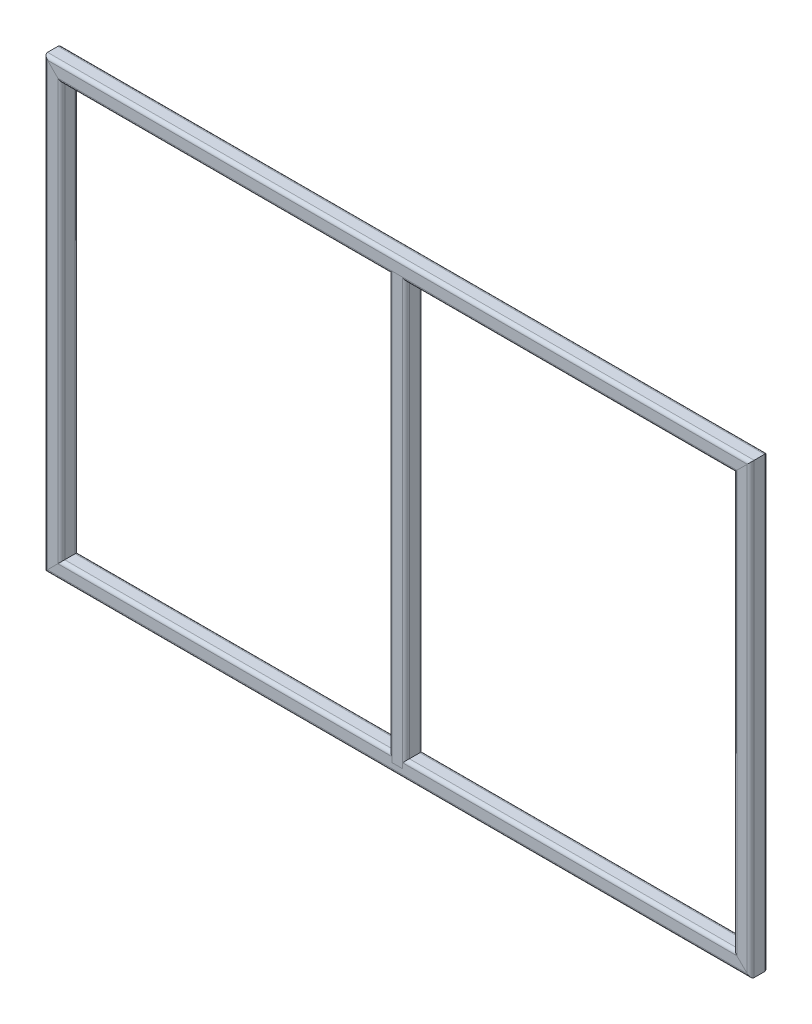
from build123d import *

# Parameters (mm, degrees)
SQUARE_TUBE_20_X_20_X_2_1_DEPTH      = 815.142135624
SQUARE_TUBE_20_X_20_X_2_1_DEPTH_BACK = 15.142135624
SQUARE_TUBE_20_X_20_X_2_1_2_DEPTH    = 530.284271247
SQUARE_TUBE_20_X_20_X_2_1_3_DEPTH    = 830.284271247
SQUARE_TUBE_20_X_20_X_2_1_4_DEPTH    = 530.284271247
SQUARE_TUBE_20_X_20_X_2_2_DEPTH      = 500


with BuildPart() as part:
    # Sketch1 → Square tube 20 X 20 X 2(1) (new, two sides: drawn at the far end of the back side and taken through both)
    with BuildSketch(Plane(origin=(-400, 250, 0), x_dir=(0, 1, 0), z_dir=(1, 0, 0)).offset(-SQUARE_TUBE_20_X_20_X_2_1_DEPTH_BACK)):
        with BuildLine():
            Line((-6, -10), (6, -10))
            ThreePointArc((6, -10), (8.828427125, -8.828427125), (10, -6))
            Line((10, -6), (10, 6))
            ThreePointArc((10, 6), (8.828427125, 8.828427125), (6, 10))
            Line((6, 10), (-6, 10))
            ThreePointArc((-6, 10), (-8.828427125, 8.828427125), (-10, 6))
            Line((-10, 6), (-10, -6))
            ThreePointArc((-10, -6), (-8.828427125, -8.828427125), (-6, -10))
        make_face()
        with BuildLine():
            Line((-6, -8), (6, -8))
            ThreePointArc((6, -8), (7.414213562, -7.414213562), (8, -6))
            Line((8, -6), (8, 6))
            ThreePointArc((8, 6), (7.414213562, 7.414213562), (6, 8))
            Line((6, 8), (-6, 8))
            ThreePointArc((-6, 8), (-7.414213562, 7.414213562), (-8, 6))
            Line((-8, 6), (-8, -6))
            ThreePointArc((-8, -6), (-7.414213562, -7.414213562), (-6, -8))
        make_face(mode=Mode.SUBTRACT)
    extrude(amount=SQUARE_TUBE_20_X_20_X_2_1_DEPTH + SQUARE_TUBE_20_X_20_X_2_1_DEPTH_BACK)

    # Square tube 20 X 20 X 2(1) mitre 1
    split(bisect_by=Plane(origin=(-400, 250, 0), x_dir=(-0.707106781, 0.707106781, 0), z_dir=(0.707106781, 0.707106781, 0)), keep=Keep.TOP)

    # Square tube 20 X 20 X 2(1) mitre 2
    split(bisect_by=Plane(origin=(400, 250, 0), x_dir=(-0.707106781, -0.707106781, 0), z_dir=(-0.707106781, 0.707106781, 0)), keep=Keep.TOP)


with BuildPart() as body_2:
    # Sketch1 on segment 2 (carried to segment 2) → Square tube 20 X 20 X 2_1 2 (new body)
    with BuildSketch(Plane(origin=(400, 265.142135624, 0), x_dir=(1, 0, 0), z_dir=(0, -1, 0))):
        with BuildLine():
            Line((-6, -10), (6, -10))
            ThreePointArc((6, -10), (8.828427125, -8.828427125), (10, -6))
            Line((10, -6), (10, 6))
            ThreePointArc((10, 6), (8.828427125, 8.828427125), (6, 10))
            Line((6, 10), (-6, 10))
            ThreePointArc((-6, 10), (-8.828427125, 8.828427125), (-10, 6))
            Line((-10, 6), (-10, -6))
            ThreePointArc((-10, -6), (-8.828427125, -8.828427125), (-6, -10))
        make_face()
        with BuildLine():
            Line((-6, -8), (6, -8))
            ThreePointArc((6, -8), (7.414213562, -7.414213562), (8, -6))
            Line((8, -6), (8, 6))
            ThreePointArc((8, 6), (7.414213562, 7.414213562), (6, 8))
            Line((6, 8), (-6, 8))
            ThreePointArc((-6, 8), (-7.414213562, 7.414213562), (-8, 6))
            Line((-8, 6), (-8, -6))
            ThreePointArc((-8, -6), (-7.414213562, -7.414213562), (-6, -8))
        make_face(mode=Mode.SUBTRACT)
    extrude(amount=SQUARE_TUBE_20_X_20_X_2_1_2_DEPTH)

    # Square tube 20 X 20 X 2_1 2 mitre 1
    split(bisect_by=Plane(origin=(400, 250, 0), x_dir=(0.707106781, 0.707106781, 0), z_dir=(0.707106781, -0.707106781, 0)), keep=Keep.TOP)

    # Square tube 20 X 20 X 2_1 2 mitre 2
    split(bisect_by=Plane(origin=(400, -250, 0), x_dir=(-0.707106781, 0.707106781, 0), z_dir=(0.707106781, 0.707106781, 0)), keep=Keep.TOP)


with BuildPart() as body_3:
    # Sketch1 on segment 3 (carried to segment 3) → Square tube 20 X 20 X 2_1 3 (new body)
    with BuildSketch(Plane(origin=(415.142135624, -250, 0), x_dir=(0, -1, 0), z_dir=(-1, 0, 0))):
        with BuildLine():
            Line((-6, -10), (6, -10))
            ThreePointArc((6, -10), (8.828427125, -8.828427125), (10, -6))
            Line((10, -6), (10, 6))
            ThreePointArc((10, 6), (8.828427125, 8.828427125), (6, 10))
            Line((6, 10), (-6, 10))
            ThreePointArc((-6, 10), (-8.828427125, 8.828427125), (-10, 6))
            Line((-10, 6), (-10, -6))
            ThreePointArc((-10, -6), (-8.828427125, -8.828427125), (-6, -10))
        make_face()
        with BuildLine():
            Line((-6, -8), (6, -8))
            ThreePointArc((6, -8), (7.414213562, -7.414213562), (8, -6))
            Line((8, -6), (8, 6))
            ThreePointArc((8, 6), (7.414213562, 7.414213562), (6, 8))
            Line((6, 8), (-6, 8))
            ThreePointArc((-6, 8), (-7.414213562, 7.414213562), (-8, 6))
            Line((-8, 6), (-8, -6))
            ThreePointArc((-8, -6), (-7.414213562, -7.414213562), (-6, -8))
        make_face(mode=Mode.SUBTRACT)
    extrude(amount=SQUARE_TUBE_20_X_20_X_2_1_3_DEPTH)

    # Square tube 20 X 20 X 2_1 3 mitre 1
    split(bisect_by=Plane(origin=(-400, -250, 0), x_dir=(0.707106781, 0.707106781, 0), z_dir=(0.707106781, -0.707106781, 0)), keep=Keep.TOP)

    # Square tube 20 X 20 X 2_1 3 mitre 2
    split(bisect_by=Plane(origin=(400, -250, 0), x_dir=(0.707106781, -0.707106781, 0), z_dir=(-0.707106781, -0.707106781, 0)), keep=Keep.TOP)


with BuildPart() as body_4:
    # Sketch1 on segment 4 (carried to segment 4) → Square tube 20 X 20 X 2_1 4 (new body)
    with BuildSketch(Plane(origin=(-400, -265.142135624, 0), x_dir=(-1, 0, 0), z_dir=(0, 1, 0))):
        with BuildLine():
            Line((-6, -10), (6, -10))
            ThreePointArc((6, -10), (8.828427125, -8.828427125), (10, -6))
            Line((10, -6), (10, 6))
            ThreePointArc((10, 6), (8.828427125, 8.828427125), (6, 10))
            Line((6, 10), (-6, 10))
            ThreePointArc((-6, 10), (-8.828427125, 8.828427125), (-10, 6))
            Line((-10, 6), (-10, -6))
            ThreePointArc((-10, -6), (-8.828427125, -8.828427125), (-6, -10))
        make_face()
        with BuildLine():
            Line((-6, -8), (6, -8))
            ThreePointArc((6, -8), (7.414213562, -7.414213562), (8, -6))
            Line((8, -6), (8, 6))
            ThreePointArc((8, 6), (7.414213562, 7.414213562), (6, 8))
            Line((6, 8), (-6, 8))
            ThreePointArc((-6, 8), (-7.414213562, 7.414213562), (-8, 6))
            Line((-8, 6), (-8, -6))
            ThreePointArc((-8, -6), (-7.414213562, -7.414213562), (-6, -8))
        make_face(mode=Mode.SUBTRACT)
    extrude(amount=SQUARE_TUBE_20_X_20_X_2_1_4_DEPTH)

    # Square tube 20 X 20 X 2_1 4 mitre 1
    split(bisect_by=Plane(origin=(-400, 250, 0), x_dir=(0.707106781, -0.707106781, 0), z_dir=(-0.707106781, -0.707106781, 0)), keep=Keep.TOP)

    # Square tube 20 X 20 X 2_1 4 mitre 2
    split(bisect_by=Plane(origin=(-400, -250, 0), x_dir=(-0.707106781, -0.707106781, 0), z_dir=(-0.707106781, 0.707106781, 0)), keep=Keep.TOP)


with BuildPart() as body_5:
    # Sketch11 → Square tube 20 X 20 X 2(2) (new body)
    with BuildSketch(Plane.XZ.offset(-250)):
        with BuildLine():
            Line((-6, -10), (6, -10))
            ThreePointArc((6, -10), (8.828427125, -8.828427125), (10, -6))
            Line((10, -6), (10, 6))
            ThreePointArc((10, 6), (8.828427125, 8.828427125), (6, 10))
            Line((6, 10), (-6, 10))
            ThreePointArc((-6, 10), (-8.828427125, 8.828427125), (-10, 6))
            Line((-10, 6), (-10, -6))
            ThreePointArc((-10, -6), (-8.828427125, -8.828427125), (-6, -10))
        make_face()
        with BuildLine():
            Line((-6, -8), (6, -8))
            ThreePointArc((6, -8), (7.414213562, -7.414213562), (8, -6))
            Line((8, -6), (8, 6))
            ThreePointArc((8, 6), (7.414213562, 7.414213562), (6, 8))
            Line((6, 8), (-6, 8))
            ThreePointArc((-6, 8), (-7.414213562, 7.414213562), (-8, 6))
            Line((-8, 6), (-8, -6))
            ThreePointArc((-8, -6), (-7.414213562, -7.414213562), (-6, -8))
        make_face(mode=Mode.SUBTRACT)
    extrude(amount=SQUARE_TUBE_20_X_20_X_2_2_DEPTH)


solid = Compound([part.part, body_2.part, body_3.part, body_4.part, body_5.part])
